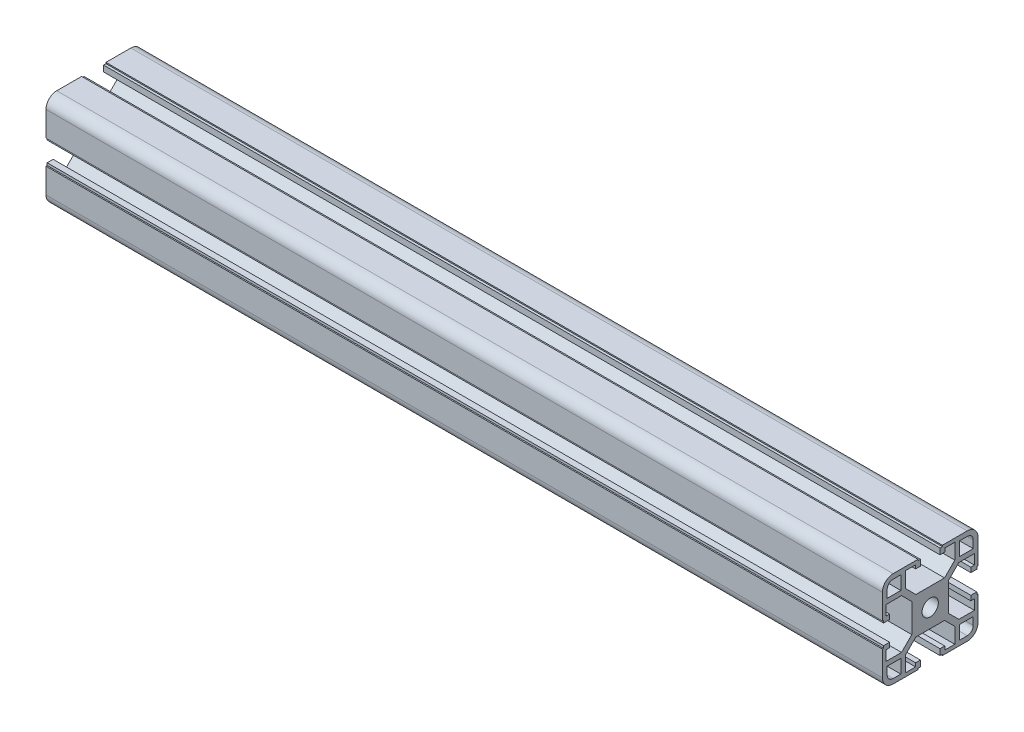
from build123d import *

# Parameters (mm, degrees)
SKETCH1_R                                 = 3.4
ALUMINIUM_PROFILE_40_X_40B_X_R4_5_1_DEPTH = 350


with BuildPart() as part:
    # Sketch1 → Aluminium profile 40 X 40B X R4.5(1) (new body)
    with BuildSketch(Plane.YZ.offset(-984.974958264)):
        with BuildLine():
            Line((-5.1, 20), (-5.1, 19.5))
            Line((-5.1, 19.5), (-4.1, 19.5))
            Line((-4.1, 19.5), (-4.1, 17))
            Line((-4.1, 17), (-6.1, 17))
            Line((-6.1, 17), (-6.1, 18.5))
            Line((-6.1, 18.5), (-10.3, 18.5))
            Line((-10.3, 18.5), (-10.3, 12))
            Line((-10.3, 12), (-6, 7.7))
            Line((-6, 7.7), (6, 7.7))
            Line((6, 7.7), (10.3, 12))
            Line((10.3, 12), (10.3, 18.5))
            Line((10.3, 18.5), (6.1, 18.5))
            Line((6.1, 18.5), (6.1, 17))
            Line((6.1, 17), (4.1, 17))
            Line((4.1, 17), (4.1, 19.5))
            Line((4.1, 19.5), (5.1, 19.5))
            Line((5.1, 19.5), (5.1, 20))
            Line((5.1, 20), (15.5, 20))
            ThreePointArc((15.5, 20), (18.681980515, 18.681980515), (20, 15.5))
            Line((20, 15.5), (20, 5.1))
            Line((20, 5.1), (19.5, 5.1))
            Line((19.5, 5.1), (19.5, 4.1))
            Line((19.5, 4.1), (17, 4.1))
            Line((17, 4.1), (17, 6.1))
            Line((17, 6.1), (18.5, 6.1))
            Line((18.5, 6.1), (18.5, 10.3))
            Line((18.5, 10.3), (12, 10.3))
            Line((12, 10.3), (7.7, 6))
            Line((7.7, 6), (7.7, -6))
            Line((7.7, -6), (12, -10.3))
            Line((12, -10.3), (18.5, -10.3))
            Line((18.5, -10.3), (18.5, -6.1))
            Line((18.5, -6.1), (17, -6.1))
            Line((17, -6.1), (17, -4.1))
            Line((17, -4.1), (19.5, -4.1))
            Line((19.5, -4.1), (19.5, -5.1))
            Line((19.5, -5.1), (20, -5.1))
            Line((20, -5.1), (20, -15.5))
            ThreePointArc((20, -15.5), (18.681980515, -18.681980515), (15.5, -20))
            Line((15.5, -20), (5.1, -20))
            Line((5.1, -20), (5.1, -19.5))
            Line((5.1, -19.5), (4.1, -19.5))
            Line((4.1, -19.5), (4.1, -17))
            Line((4.1, -17), (6.1, -17))
            Line((6.1, -17), (6.1, -18.5))
            Line((6.1, -18.5), (10.3, -18.5))
            Line((10.3, -18.5), (10.3, -12))
            Line((10.3, -12), (6, -7.7))
            Line((6, -7.7), (-6, -7.7))
            Line((-6, -7.7), (-10.3, -12))
            Line((-10.3, -12), (-10.3, -18.5))
            Line((-10.3, -18.5), (-6.1, -18.5))
            Line((-6.1, -18.5), (-6.1, -17))
            Line((-6.1, -17), (-4.1, -17))
            Line((-4.1, -17), (-4.1, -19.5))
            Line((-4.1, -19.5), (-5.1, -19.5))
            Line((-5.1, -19.5), (-5.1, -20))
            Line((-5.1, -20), (-15.5, -20))
            ThreePointArc((-15.5, -20), (-18.681980515, -18.681980515), (-20, -15.5))
            Line((-20, -15.5), (-20, -5.1))
            Line((-20, -5.1), (-19.5, -5.1))
            Line((-19.5, -5.1), (-19.5, -4.1))
            Line((-19.5, -4.1), (-17, -4.1))
            Line((-17, -4.1), (-17, -6.1))
            Line((-17, -6.1), (-18.5, -6.1))
            Line((-18.5, -6.1), (-18.5, -10.3))
            Line((-18.5, -10.3), (-12, -10.3))
            Line((-12, -10.3), (-7.7, -6))
            Line((-7.7, -6), (-7.7, 6))
            Line((-7.7, 6), (-12, 10.3))
            Line((-12, 10.3), (-18.5, 10.3))
            Line((-18.5, 10.3), (-18.5, 6.1))
            Line((-18.5, 6.1), (-17, 6.1))
            Line((-17, 6.1), (-17, 4.1))
            Line((-17, 4.1), (-19.5, 4.1))
            Line((-19.5, 4.1), (-19.5, 5.1))
            Line((-19.5, 5.1), (-20, 5.1))
            Line((-20, 5.1), (-20, 15.5))
            ThreePointArc((-20, 15.5), (-18.681980515, 18.681980515), (-15.5, 20))
            Line((-15.5, 20), (-5.1, 20))
        make_face()
        Circle(SKETCH1_R, mode=Mode.SUBTRACT)
        with BuildLine():
            Line((12.3, 18), (15.5, 18))
            ThreePointArc((15.5, 18), (17.267766953, 17.267766953), (18, 15.5))
            Line((18, 15.5), (18, 12.3))
            Line((18, 12.3), (12.3, 12.3))
            Line((12.3, 12.3), (12.3, 18))
        make_face(mode=Mode.SUBTRACT)
        with BuildLine():
            Line((-15.5, 18), (-12.3, 18))
            Line((-12.3, 18), (-12.3, 12.3))
            Line((-12.3, 12.3), (-18, 12.3))
            Line((-18, 12.3), (-18, 15.5))
            ThreePointArc((-18, 15.5), (-17.267766953, 17.267766953), (-15.5, 18))
        make_face(mode=Mode.SUBTRACT)
        with BuildLine():
            Line((-18, -12.3), (-12.3, -12.3))
            Line((-12.3, -12.3), (-12.3, -18))
            Line((-12.3, -18), (-15.5, -18))
            ThreePointArc((-15.5, -18), (-17.267766953, -17.267766953), (-18, -15.5))
            Line((-18, -15.5), (-18, -12.3))
        make_face(mode=Mode.SUBTRACT)
        with BuildLine():
            Line((12.3, -12.3), (18, -12.3))
            Line((18, -12.3), (18, -15.5))
            ThreePointArc((18, -15.5), (17.267766953, -17.267766953), (15.5, -18))
            Line((15.5, -18), (12.3, -18))
            Line((12.3, -18), (12.3, -12.3))
        make_face(mode=Mode.SUBTRACT)
    extrude(amount=ALUMINIUM_PROFILE_40_X_40B_X_R4_5_1_DEPTH)


solid = part.part
